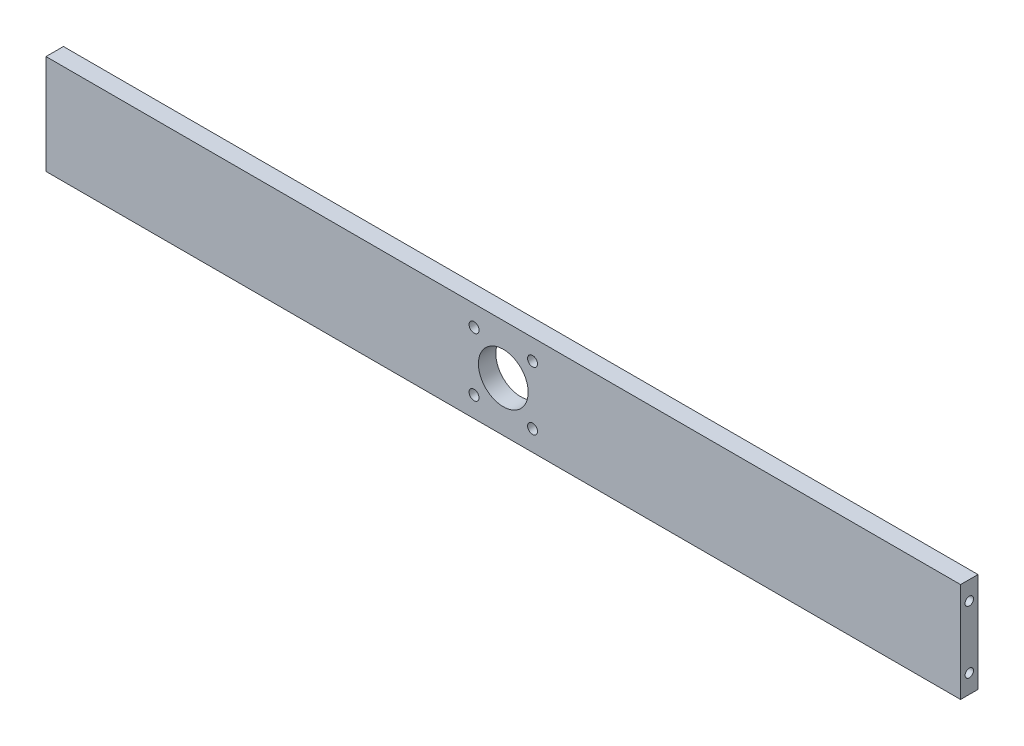
SolidWorks part; units mm, degrees
material "普通碳钢"
ref_plane "Front Plane" through (0, 0, 0) normal (0, 0, 1) x (1, 0, 0)
ref_plane "Top Plane" through (0, 0, 0) normal (0, 1, 0) x (1, 0, 0)
ref_plane "Right Plane" through (0, 0, 0) normal (1, 0, 0) x (0, 0, -1)
sketch "Sketch1" plane through (0, 0, 0) normal (0, 0, 1) x (1, 0, 0)
  line L1 (0, 0) -> (735, 0)
  line L2 (0, 0) -> (0, 80)
  line L3 (0, 80) -> (735, 80)
  line L4 (735, 0) -> (735, 80)
  dimension "D1" = 735
  dimension "D2" = 80
extrude "Boss-Extrude1" add sketch "Sketch1" along normal blind 14
sketch "Sketch2" plane through (0, 0, 14) normal (0, 0, 1) x (1, 0, 0)
  line L0 (344, 63.5) -> (391, 63.5) construction
  line L1 (391, 63.5) -> (391, 16.5) construction
  line L2 (391, 16.5) -> (344, 16.5) construction
  line L3 (344, 16.5) -> (344, 63.5) construction
  line L4 (367.5, 63.5) -> (367.5, 80) construction
  line L5 (735, 80) -> (0, 80) construction
  line L6 (344, 40) -> (0, 40) construction
  line L7 (0, 80) -> (0, 0) construction
  line L8 (367.5, 40) -> (367.5, 63.5) construction
  line L9 (367.5, 40) -> (344, 40) construction
  circle A0 centre (344, 63.5) radius 4
  circle A1 centre (344, 16.5) radius 4
  circle A2 centre (391, 16.5) radius 4
  circle A3 centre (391, 63.5) radius 4
  circle A4 centre (367.5, 40) radius 20
  circle A5 centre (12.5, 65) radius 5 construction
  circle A6 centre (12.5, 15) radius 5 construction
  circle A7 centre (722.5, 65) radius 5 construction
  circle A8 centre (722.5, 15) radius 5 construction
  dimension "D1" = 8
  dimension "D2" = 40
  dimension "D5" = 12.5
  dimension "D7" = 10
  dimension "D3" = 47
  dimension "D4" = 47
  dimension "D6" = 50
extrude "Cut-Extrude1" cut sketch "Sketch2" against normal blind 14
hole_wizard "M8 Tapped Hole1" positions "3DSketch1" profile "Sketch3" tap size "M8" standard "GB"
sketch3d "3DSketch1"
  line L0 (0, 80, 7) -> (0, 65, 7) construction
  line L1 (0, 80, 14) -> (0, 80, 0) construction
  line L2 (0, 65, 7) -> (0, 15, 7) construction
  line L4 (0, 40, 7) -> (0, 40, 14) construction
  line L5 (0, 80, 14) -> (0, 0, 14) construction
  point P0 (0, 65, 7)
  point P2 (0, 15, 7)
  dimension "D1" = 50
sketch "Sketch3" plane through (0, 65, 7) normal (0, 1, 0) x (0, 0, 1)
  line L0 (0, 0) -> (0, 21.7929)
  line L1 (0, 21.7929) -> (3.4, 19.75)
  line L2 (3.4, 19.75) -> (3.4, 0)
  line L5 (3.4, 0) -> (0, 0)
  line L10 (0, 21.7929) -> (-3.4, 19.75) construction
  line L11 (0, -6.35) -> (0, 107.95) construction
  dimension "螺纹孔钻头直径" = 6.8
  dimension "螺纹孔钻头深度" = 19.75
  dimension "导头角度" = 118
cosmetic thread "Hole Cosmetic Thread1" parameters "D1"=16, "D2"=8
cosmetic thread "Hole Cosmetic Thread2" parameters "D1"=16, "D2"=8
hole_wizard "M8 Tapped Hole2" positions "3DSketch2" profile "Sketch4" tap size "M8" standard "GB"
sketch3d "3DSketch2"
  line L0 (735, 0, 7) -> (735, 15, 7) construction
  line L1 (735, 0, 14) -> (735, 0, 0) construction
  line L2 (735, 15, 7) -> (735, 65, 7) construction
  line L4 (735, 40, 7) -> (735, 40, 14) construction
  line L5 (735, 0, 14) -> (735, 80, 14) construction
  point P0 (735, 15, 7)
  point P2 (735, 65, 7)
  dimension "D1" = 50
sketch "Sketch4" plane through (735, 15, 7) normal (0, 1, 0) x (0, 0, -1)
  line L0 (0, 0) -> (0, 21.7929)
  line L1 (0, 21.7929) -> (3.4, 19.75)
  line L2 (3.4, 19.75) -> (3.4, 0)
  line L5 (3.4, 0) -> (0, 0)
  line L10 (0, 21.7929) -> (-3.4, 19.75) construction
  line L11 (0, -6.35) -> (0, 107.95) construction
  dimension "螺纹孔钻头直径" = 6.8
  dimension "螺纹孔钻头深度" = 19.75
  dimension "导头角度" = 118
cosmetic thread "Hole Cosmetic Thread3" parameters "D1"=16, "D2"=8
cosmetic thread "Hole Cosmetic Thread4" parameters "D1"=16, "D2"=8
